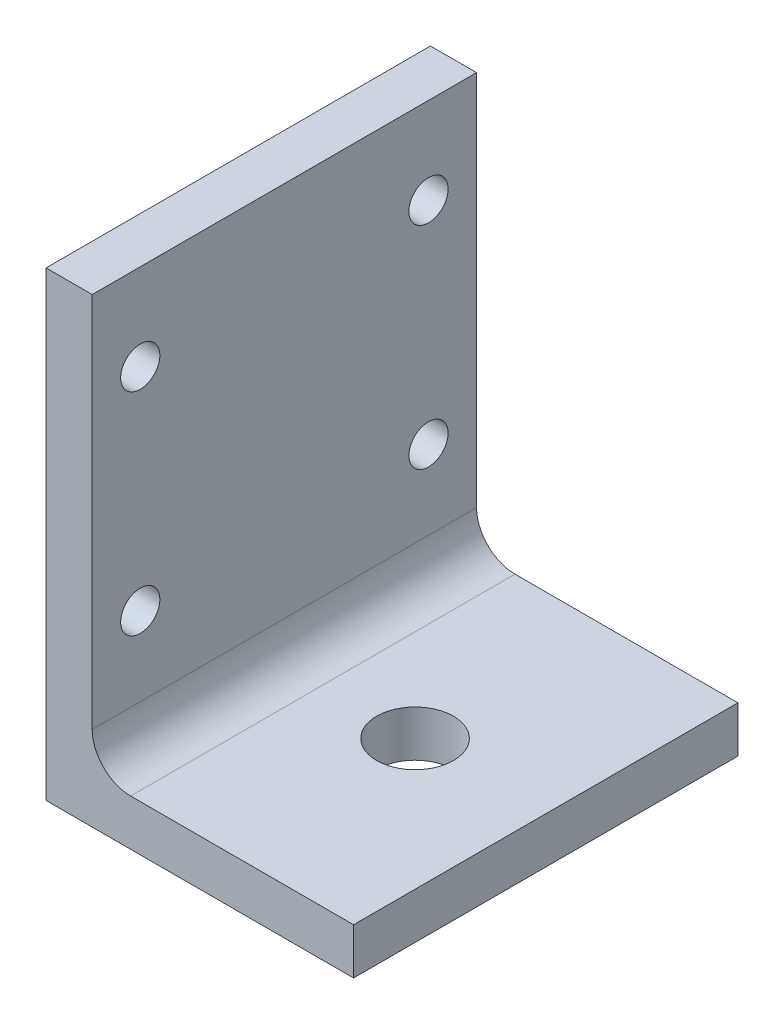
from build123d import *

# Parameters (mm, degrees)
BOSS_EXTRUDE1_DEPTH    = 100
M12_TAPPED_HOLE1_D     = 10.2
M12_TAPPED_HOLE1_DEPTH = 29.25
M12_TAPPED_HOLE1_TIP   = 3.064389157
SKETCH5_R              = 10
CUT_EXTRUDE1_DEPTH     = 100


with BuildPart() as part:
    # Sketch1 → Boss-Extrude1 (new body)
    with BuildSketch(Plane.XY):
        with BuildLine():
            Line((0, 0), (0, -120))
            Line((0, -120), (80, -120))
            Line((80, -120), (80, -108))
            Line((80, -108), (22, -108))
            ThreePointArc((22, -108), (14.928932188, -105.071067812), (12, -98))
            Line((12, -98), (12, 0))
            Line((12, 0), (0, 0))
        make_face()
    extrude(amount=BOSS_EXTRUDE1_DEPTH)

    # M12 Tapped Hole1
    with Locations(Plane(origin=(12, 0, 0), x_dir=(0, 0, -1), z_dir=(1, 0, 0))):
        with Locations((-87.5, -22.5), (-12.5, -22.5), (-12.5, -77.5), (-87.5, -77.5)):
            Hole(M12_TAPPED_HOLE1_D / 2, depth=M12_TAPPED_HOLE1_DEPTH)
            with Locations((0, 0, -(M12_TAPPED_HOLE1_DEPTH + M12_TAPPED_HOLE1_TIP / 2))):  # 118° drill point
                Cone(0, M12_TAPPED_HOLE1_D / 2, M12_TAPPED_HOLE1_TIP, mode=Mode.SUBTRACT)

    # Sketch5 → Cut-Extrude1 (cut)
    with BuildSketch(Plane(origin=(0, -108, 0), x_dir=(1, 0, 0), z_dir=(0, 1, 0))):
        with Locations(Location((46, -50, 0), (0, 0, 270))):
            Circle(SKETCH5_R)
    extrude(amount=-CUT_EXTRUDE1_DEPTH, mode=Mode.SUBTRACT)


solid = part.part
